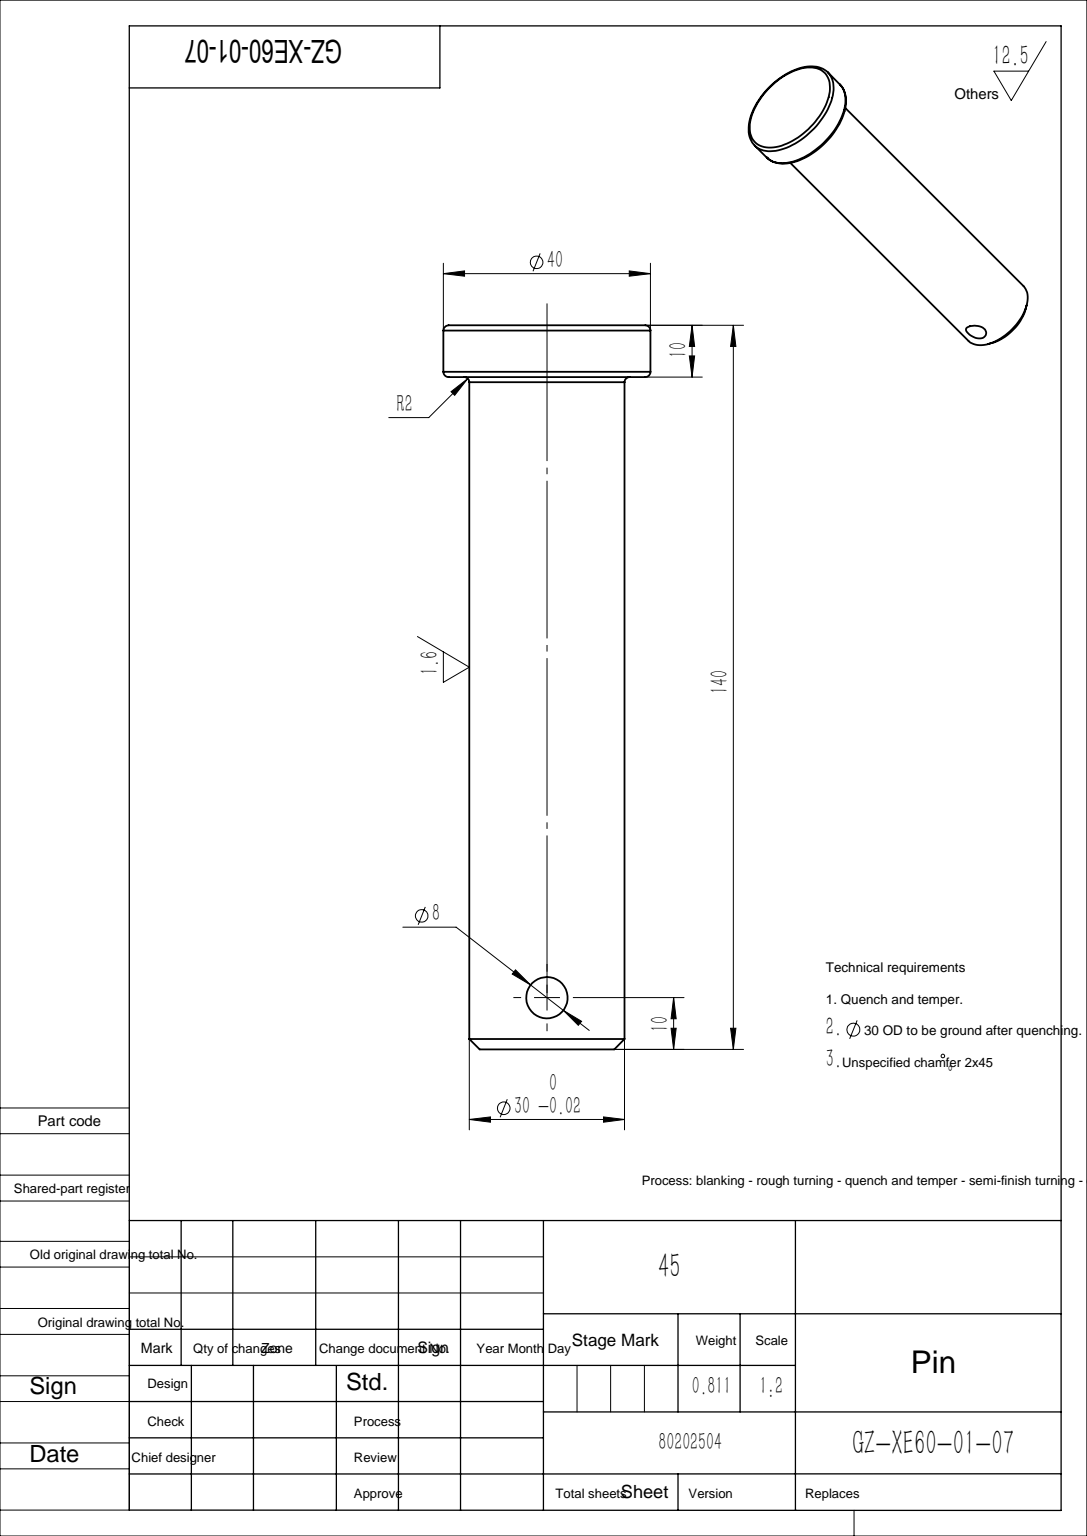
from build123d import *

# Parameters (mm, degrees)
SKETCH1_R               = 15
BOSS_EXTRUDE1_DEPTH     = 130
SKETCH2_R               = 20
BOSS_EXTRUDE2_DEPTH     = 10
CUT_EXTRUDE1_DEPTH      = 143.828568571
CUT_EXTRUDE1_DEPTH_BACK = 143.828568571
SKETCH3_R               = 4
CHAMFER1_SIZE           = 2
FILLET1_R               = 1
FILLET2_R               = 1


with BuildPart() as part:
    # Sketch1 → Boss-Extrude1 (new body)
    with BuildSketch(Plane.XY):
        Circle(SKETCH1_R)
    extrude(amount=BOSS_EXTRUDE1_DEPTH)

    # Sketch2 → Boss-Extrude2 (add)
    with BuildSketch(Plane.XY.offset(130)):
        Circle(SKETCH2_R)
    extrude(amount=BOSS_EXTRUDE2_DEPTH)

    # Sketch3 → Cut-Extrude1 (cut, two sides: drawn at the far end of the back side and taken through both)
    with BuildSketch(Plane(origin=(0, 0, 0), x_dir=(1, 0, 0), z_dir=(0, 1, 0)).offset(-CUT_EXTRUDE1_DEPTH_BACK)):
        with Locations(Location((0, -10, 0), (0, 0, 270))):
            Circle(SKETCH3_R)
    extrude(amount=CUT_EXTRUDE1_DEPTH + CUT_EXTRUDE1_DEPTH_BACK, mode=Mode.SUBTRACT)

    # Chamfer1
    chamfer1_edges = [part.edges().sort_by_distance(p)[0] for p in [
        (-15, 0, 0),
    ]]
    chamfer(chamfer1_edges, length=CHAMFER1_SIZE)

    # Fillet1
    fillet1_edges = [part.edges().sort_by_distance(p)[0] for p in [
        (-15, 0, 130),
    ]]
    fillet(fillet1_edges, radius=FILLET1_R)

    # Fillet2
    fillet2_edges = [part.edges().sort_by_distance(p)[0] for p in [
        (-20, 0, 130),
        (-20, 0, 140),
    ]]
    fillet(fillet2_edges, radius=FILLET2_R)


solid = part.part
